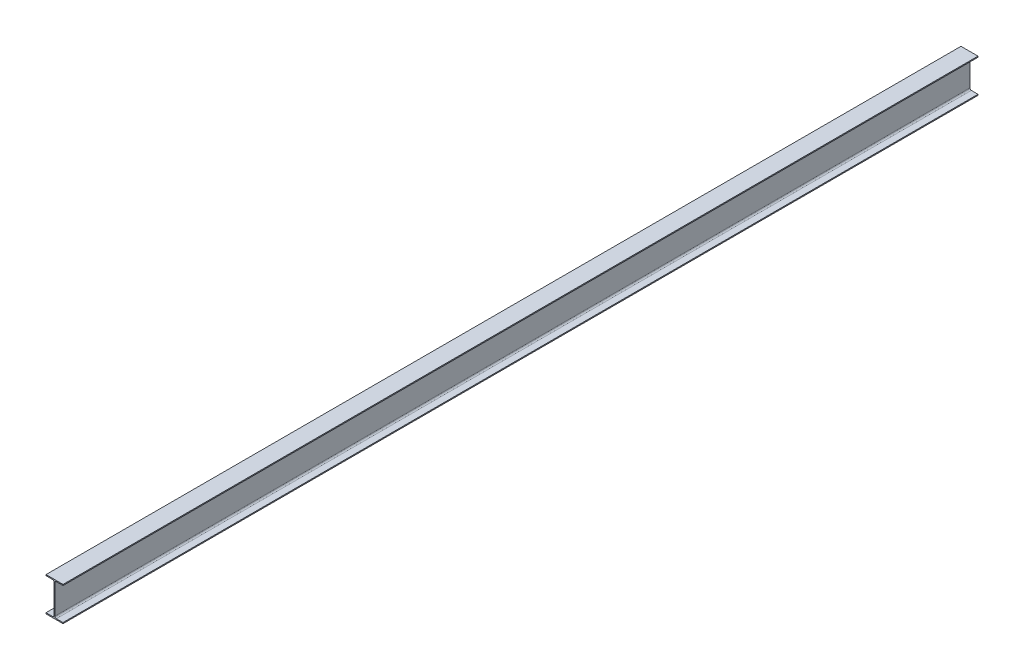
from build123d import *

# Parameters (mm, degrees)
BOSS_EXTRUDE1_DEPTH = 8060


with BuildPart() as part:
    # Sketch1 → Boss-Extrude1 (new body)
    with BuildSketch(Plane.XY):
        with BuildLine():
            Line((75, 0), (-75, 0))
            Line((-75, 0), (-75, 9))
            Line((-75, 9), (-16.25, 9))
            ThreePointArc((-16.25, 9), (-7.057611845, 12.807611845), (-3.25, 22))
            Line((-3.25, 22), (-3.25, 278))
            ThreePointArc((-3.25, 278), (-7.057611845, 287.192388155), (-16.25, 291))
            Line((-16.25, 291), (-75, 291))
            Line((-75, 291), (-75, 300))
            Line((-75, 300), (75, 300))
            Line((75, 300), (75, 291))
            Line((75, 291), (16.25, 291))
            ThreePointArc((16.25, 291), (7.057611845, 287.192388155), (3.25, 278))
            Line((3.25, 278), (3.25, 22))
            ThreePointArc((3.25, 22), (7.057611845, 12.807611845), (16.25, 9))
            Line((16.25, 9), (75, 9))
            Line((75, 9), (75, 0))
        make_face()
    extrude(amount=BOSS_EXTRUDE1_DEPTH)


solid = part.part
